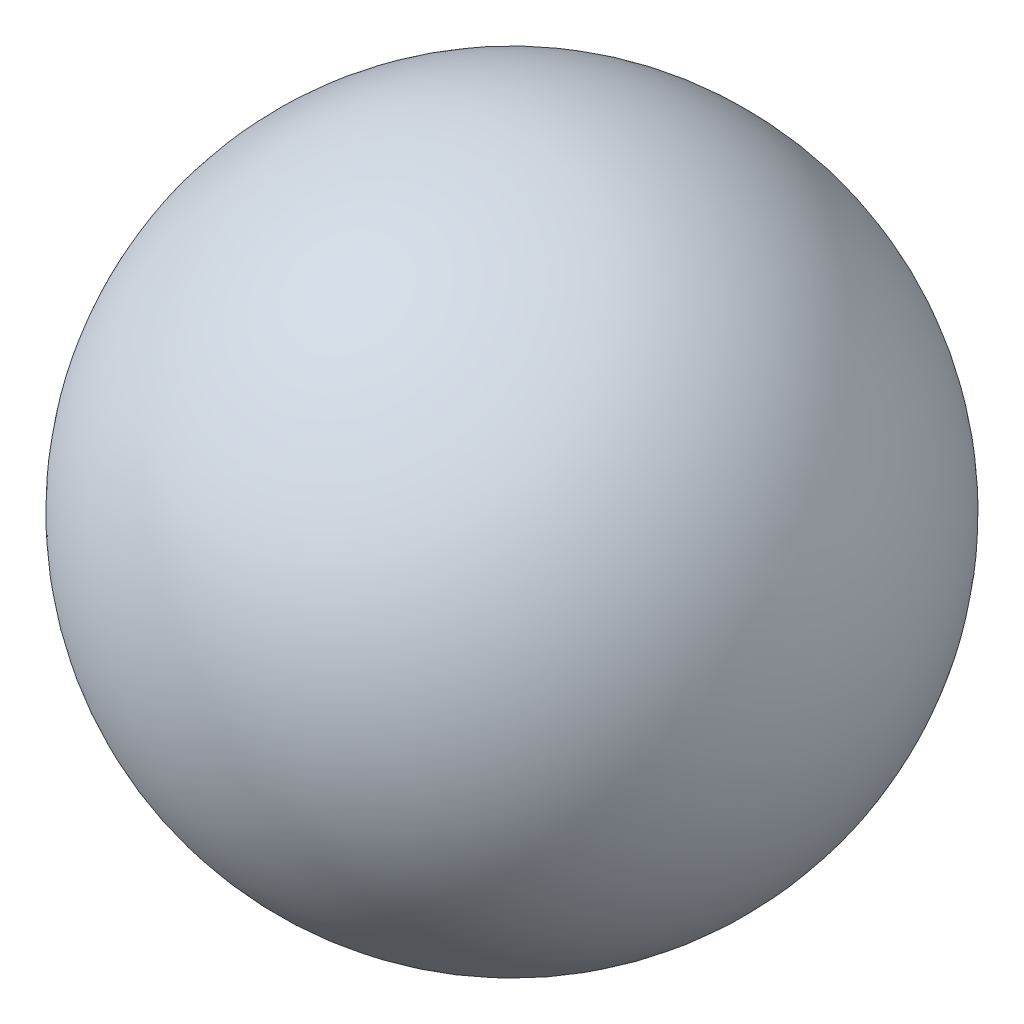
from build123d import *


with BuildPart() as part:
    # Sketch1 → Revolve1 (revolve)
    with BuildSketch(Plane.XY):
        with BuildLine():
            Line((29.4, 0), (43.1, 0))
            ThreePointArc((43.1, 0), (36.25, 6.85), (29.4, 0))
        make_face()
    revolve(axis=Axis((0, 0, 0), (1, 0, 0)))


solid = part.part
